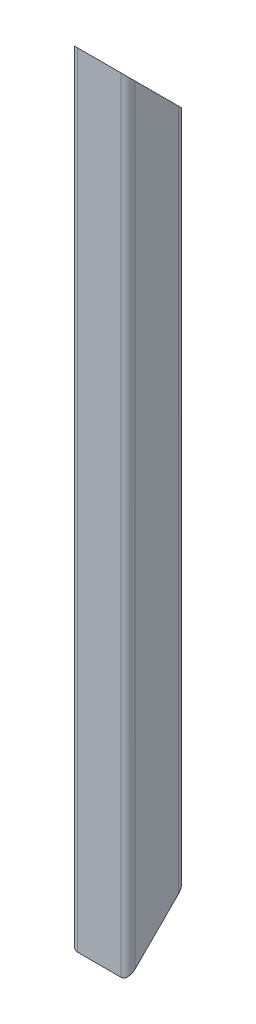
SolidWorks part; units mm, degrees
ref_plane "Front" through (0, 0, 0) normal (0, 0, 1) x (1, 0, 0)
ref_plane "Top" through (0, 0, 0) normal (0, 1, 0) x (1, 0, 0)
ref_plane "Right" through (0, 0, 0) normal (1, 0, 0) x (0, 0, -1)
sketch "草图1" plane through (0, 0, 0) normal (0, 1, 0) x (1, 0, 0)
  line L0 (-19, -7.2781) -> (19, -7.2781)
  line L1 (-19, -12.2781) -> (19, -12.2781)
  line L2 (-25, -6.2781) -> (-25, 31.7219)
  line L3 (-19, 37.7219) -> (19, 37.7219)
  line L4 (25, -6.2781) -> (25, 31.7219)
  line L5 (20, -6.2781) -> (20, 31.7219)
  line L6 (-19, 32.7219) -> (19, 32.7219)
  line L11 (-20, -6.2781) -> (-20, 31.7219)
  arc A0 (-19, -12.2781) -> (-25, -6.2781) centre (-19, -6.2781) cw
  arc A1 (19, -12.2781) -> (25, -6.2781) centre (19, -6.2781) ccw
  arc A2 (19, 37.7219) -> (25, 31.7219) centre (19, 31.7219) cw
  arc A3 (-25, 31.7219) -> (-19, 37.7219) centre (-19, 31.7219) cw
  arc A4 (19, -7.2781) -> (20, -6.2781) centre (19, -6.2781) ccw
  arc A5 (19, 32.7219) -> (20, 31.7219) centre (19, 31.7219) cw
  arc A6 (-20, 31.7219) -> (-19, 32.7219) centre (-19, 31.7219) cw
  arc A7 (-19, -7.2781) -> (-20, -6.2781) centre (-19, -6.2781) cw
  point P9 (25, -12.2781)
  point P12 (25, 37.7219)
  point P15 (-25, 37.7219)
  dimension "D3" = 6
  dimension "D1" = 50
  dimension "D2" = 50
  dimension "D4" = 5
extrude "凸台-拉伸1" add sketch "草图1" along normal blind 680
sketch "草图2" plane through (25, 0, 0) normal (1, 0, 0) x (0, 0, -1)
  line L0 (-12.2781, 680) -> (37.7219, 680)
  line L1 (37.7219, 680) -> (37.7219, 630)
  line L2 (37.7219, 680) -> (37.7219, 0) construction
  line L3 (37.7219, 630) -> (-12.2781, 680)
  line L4 (-12.2781, 0) -> (37.7219, 50)
  line L5 (37.7219, 50) -> (37.7219, 0)
  line L6 (37.7219, 0) -> (-12.2781, 0)
  dimension "D1" = 45
  dimension "D2" = 45
extrude "切除-拉伸1" cut sketch "草图2" against normal through all
